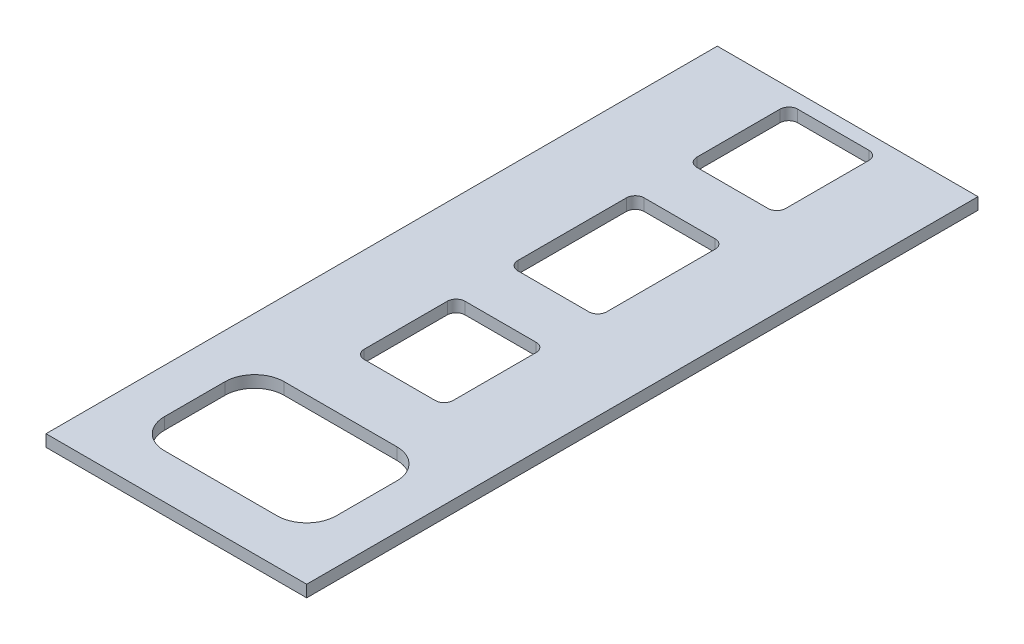
from build123d import *

# Parameters (mm, degrees)
SKETCH_1_W          = 880
SKETCH_1_H          = 2266
EXTRUDE_1_DEPTH     = 40
SKETCH_2_W          = 300
SKETCH_2_H          = 340.469439268
CUT_EXTRUDE_1_DEPTH = 1217.095802147
SKETCH_3_W          = 300
SKETCH_3_H          = 426.530560732
CUT_EXTRUDE_2_DEPTH = 1217.095802147
SKETCH_4_W          = 300
SKETCH_4_H          = 340.469439268
CUT_EXTRUDE_3_DEPTH = 1217.095802147
SKETCH_5_W          = 580
SKETCH_5_H          = 404.015280366
CUT_EXTRUDE_4_DEPTH = 1217.095802147
FILLET_2_R          = 100
FILLET_3_R          = 30


with BuildPart() as part:
    # 草图1 → 凸台-拉伸1 (new body)
    with BuildSketch(Plane(origin=(0, 0, 0), x_dir=(1, 0, 0), z_dir=(0, 1, 0))):
        Rectangle(SKETCH_1_W, SKETCH_1_H)
    extrude(amount=EXTRUDE_1_DEPTH)

    # 草图2 → 切除-拉伸1 (cut, through all)
    with BuildSketch(Plane.XZ):
        with Locations((0, 208.75)):
            Rectangle(SKETCH_2_W, SKETCH_2_H)
    extrude(amount=-CUT_EXTRUDE_1_DEPTH, mode=Mode.SUBTRACT)

    # 草图3 → 切除-拉伸2 (cut, through all)
    with BuildSketch(Plane.XZ):
        with Locations((0, -352.75)):
            Rectangle(SKETCH_3_W, SKETCH_3_H)
    extrude(amount=-CUT_EXTRUDE_2_DEPTH, mode=Mode.SUBTRACT)

    # 草图4 → 切除-拉伸3 (cut, through all)
    with BuildSketch(Plane(origin=(0, 0, 0), x_dir=(-1, 0, 0), z_dir=(0, -1, 0))):
        with Locations((0, 914.25)):
            Rectangle(SKETCH_4_W, SKETCH_4_H)
    extrude(amount=-CUT_EXTRUDE_3_DEPTH, mode=Mode.SUBTRACT)

    # 草图5 → 切除-拉伸4 (cut, through all)
    with BuildSketch(Plane.XZ):
        with Locations((0, 780.992359817)):
            Rectangle(SKETCH_5_W, SKETCH_5_H)
    extrude(amount=-CUT_EXTRUDE_4_DEPTH, mode=Mode.SUBTRACT)

    # 圆角2
    fillet_2_edges = [part.edges().sort_by_distance(p)[0] for p in [
        (-290, 20, 578.984719634),
        (-290, 20, 983),
        (290, 20, 983),
        (290, 20, 578.984719634),
    ]]
    fillet(fillet_2_edges, radius=FILLET_2_R)

    # 圆角3
    fillet_3_edges = [part.edges().sort_by_distance(p)[0] for p in [
        (-150, 20, 38.515280366),
        (-150, 20, 378.984719634),
        (150, 20, 378.984719634),
        (150, 20, 38.515280366),
        (-150, 20, -566.015280366),
        (-150, 20, -139.484719634),
        (150, 20, -139.484719634),
        (150, 20, -566.015280366),
        (-150, 20, -1084.484719634),
        (-150, 20, -744.015280366),
        (150, 20, -744.015280366),
        (150, 20, -1084.484719634),
    ]]
    fillet(fillet_3_edges, radius=FILLET_3_R)


solid = part.part
